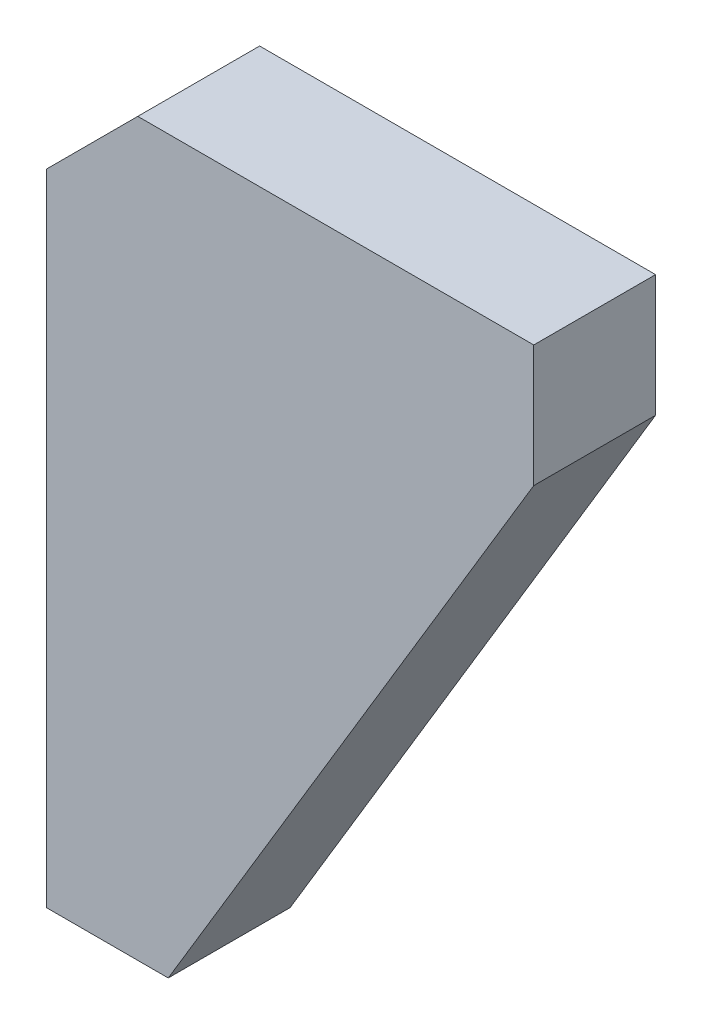
from build123d import *

# Parameters (mm, degrees)
BOSS_EXTRUDE1_DEPTH = 20


with BuildPart() as part:
    # Sketch1 → Boss-Extrude1 (new body)
    with BuildSketch(Plane.XY):
        Polygon((0, 0), (0, 105), (15, 120), (80, 120), (80, 100), (20, 0), align=None)
    extrude(amount=BOSS_EXTRUDE1_DEPTH)


solid = part.part
